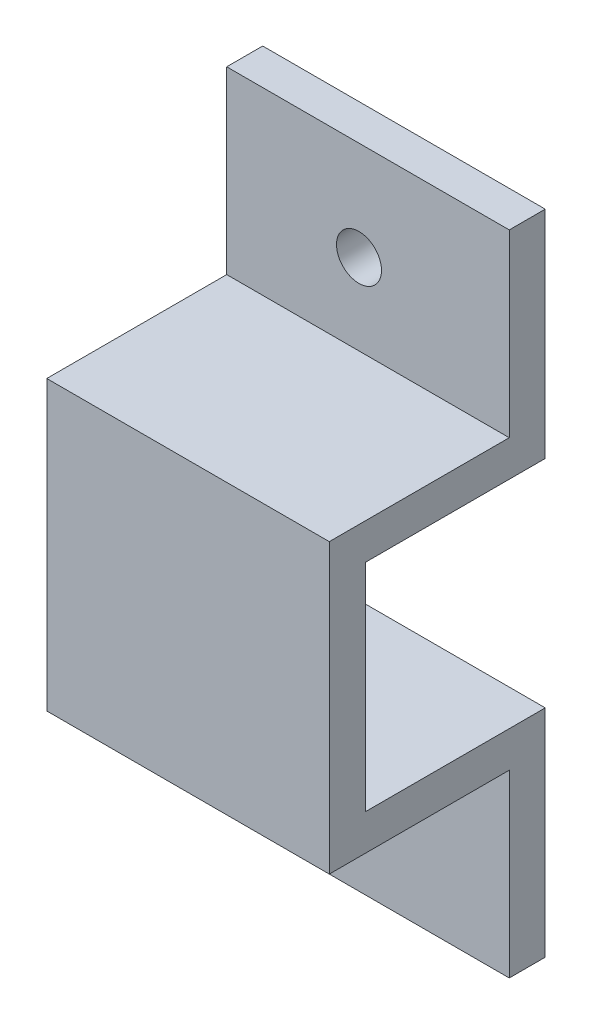
SolidWorks part; units mm, degrees
ref_plane "Front Plane" through (0, 0, 0) normal (0, 0, 1) x (1, 0, 0)
ref_plane "Top Plane" through (0, 0, 0) normal (0, 1, 0) x (1, 0, 0)
ref_plane "Right Plane" through (0, 0, 0) normal (1, 0, 0) x (0, 0, -1)
other "Configuration Table"
sketch "Sketch1" plane through (0, 0, 0) normal (0, 0, 1) x (1, 0, 0)
  line L1 (-8.35, 6) -> (8.35, 6)
  line L2 (-8.35, 6) -> (-8.35, -6)
  line L3 (-8.35, -6) -> (8.35, -6)
  line L4 (8.35, 6) -> (8.35, -6)
  line L5 (0, -6) -> (0, 6) construction
  line L6 (-8.35, 0) -> (8.35, 0) construction
  point P0 (0, 0)
  dimension "D1" = 12
  dimension "D2" = 16.7
extrude "Boss-Extrude1" add sketch "Sketch1" along normal blind 2
sketch "Sketch2" plane through (0, 0, 2) normal (0, 0, 1) x (1, 0, 0)
  line L0 (-8.35, 6) -> (8.35, 6)
  line L1 (8.35, 6) -> (8.35, 8)
  line L2 (8.35, 8) -> (-8.35, 8)
  line L3 (-8.35, 8) -> (-8.35, 6)
  line L4 (-10.9719, 0) -> (10.4384, 0) construction
  line L5 (8.35, -8) -> (-8.35, -8)
  line L6 (8.35, -6) -> (8.35, -8)
  line L7 (-8.35, -6) -> (8.35, -6)
  line L8 (-8.35, -8) -> (-8.35, -6)
  dimension "D1" = 2
extrude "Boss-Extrude2" add sketch "Sketch2" against normal blind 12
sketch "Sketch4" plane through (-8.35, 0, 0) normal (-1, 0, 0) x (0, 0, 1)
  line L0 (-10, -8) -> (-10, -18)
  line L1 (4.6478, 0) -> (-10.7567, 0) construction
  line L2 (-10, -8) -> (-8, -8)
  line L3 (-10, -8) -> (2, -8) construction
  line L4 (-10, -18) -> (-8, -18)
  line L5 (-8, -18) -> (-8, -8)
  line L6 (-10, 18) -> (-8, 18)
  line L7 (-10, 8) -> (-10, 18)
  line L8 (-10, 8) -> (-8, 8)
  line L9 (-8, 18) -> (-8, 8)
  dimension "D1" = 10
  dimension "D2" = 2
extrude "Boss-Extrude3" add sketch "Sketch4" against normal up to surface (16.7 mm away) up to face at (8.35, 0, -4.5)
sketch "Sketch5" plane through (0, 0, -8) normal (0, 0, 1) x (1, 0, 0)
  line L0 (0, 13.3964) -> (0, -13.5111) construction
  line L1 (0, 12.5) -> (6.1194, 12.5) construction
  line L2 (-11.908, 0) -> (11.8179, 0) construction
  line L3 (0, -12.5) -> (6.1194, -12.5) construction
  dimension "D1" = 12.5
hole_wizard "M3 Tapped Hole1" positions "Sketch6" profile "Sketch7" tap size "M3" standard "GB" end condition up to next
sketch "Sketch6" plane through (0, 0, -8) normal (0, 0, 1) x (1, 0, 0)
  point P0 (0, -12.5)
  point P3 (0, 12.5)
sketch "Sketch7" plane through (0, -12.5, -8) normal (1, 0, 0) x (0, -1, 0)
  line L0 (0, 0) -> (0, 2)
  line L1 (0, 2) -> (1.25, 2)
  line L2 (1.25, 2) -> (1.25, 0)
  line L5 (1.25, 0) -> (0, 0)
  line L11 (0, -6.35) -> (0, 107.95) construction
  dimension "通孔螺纹孔钻头直径" = 2.5
  dimension "通孔螺纹孔钻头深度" = 2
cosmetic thread "Hole Thread Line1" parameters "D2"=3
cosmetic thread "Hole Thread Line2" parameters "D2"=3
sketch "Sketch8" plane through (-8.35, 0, 0) normal (-1, 0, 0) x (0, 0, 1)
  line L12 (0, 6) -> (0, -6)
  line L13 (0, -6) -> (-10, -6)
  line L14 (-10, -6) -> (-10, -18)
  line L15 (-10, -18) -> (-8, -18)
  line L16 (-8, -18) -> (-8, -8)
  line L17 (-8, -8) -> (2, -8)
  line L18 (2, -8) -> (2, 8)
  line L19 (2, 8) -> (-8, 8)
  line L20 (-8, 8) -> (-8, 18)
  line L21 (-8, 18) -> (-10, 18)
  line L22 (-10, 18) -> (-10, 6)
  line L23 (-10, 6) -> (0, 6)
  line L24 (0, 6) -> (0, -6)
  line L25 (0, -6) -> (-10, -6)
  line L26 (-10, -6) -> (-10, -18)
  line L27 (-10, -18) -> (-8, -18)
  line L28 (-8, -18) -> (-8, -8)
  line L29 (-8, -8) -> (2, -8)
  line L30 (2, -8) -> (2, 8)
  line L31 (2, 8) -> (-8, 8)
  line L32 (-8, 8) -> (-8, 18)
  line L33 (-8, 18) -> (-10, 18)
  line L34 (-10, 18) -> (-10, 6)
  line L35 (-10, 6) -> (0, 6)
  dimension "D1" = 0
extrude "Cut-Extrude1" cut sketch "Sketch8" against normal blind 1
